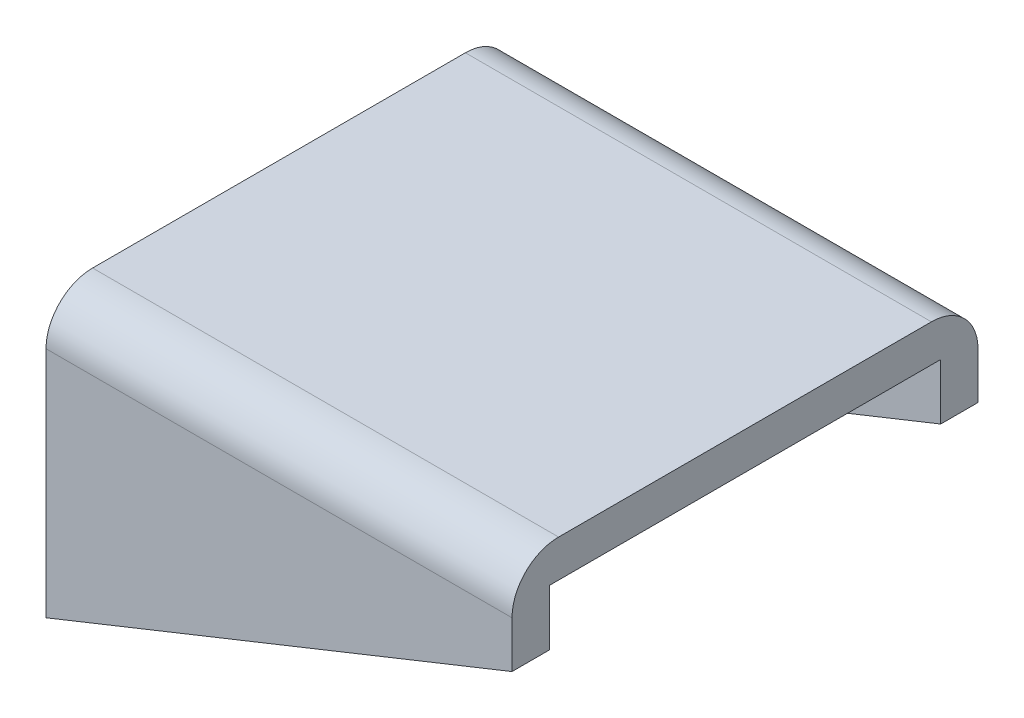
SolidWorks part; units mm, degrees
ref_plane "前视基准面" through (0, 0, 0) normal (0, 0, 1) x (1, 0, 0)
ref_plane "上视基准面" through (0, 0, 0) normal (0, 1, 0) x (1, 0, 0)
ref_plane "右视基准面" through (0, 0, 0) normal (1, 0, 0) x (0, 0, -1)
sketch "草图1" plane through (0, 0, 0) normal (0, 0, 1) x (1, 0, 0)
  line L0 (0, 0) -> (0, 60)
  line L1 (0, 60) -> (100, 60)
  line L2 (100, 60) -> (100, 40)
  line L3 (100, 40) -> (0, 0)
extrude "凸台-拉伸1" add sketch "草图1" along normal blind 100
shell "抽壳1" thickness 8
fillet "圆角1" radius 10 1 edges at (50, 60, 100)
fillet "圆角2" radius 10 1 edges at (50, 60, 0)
